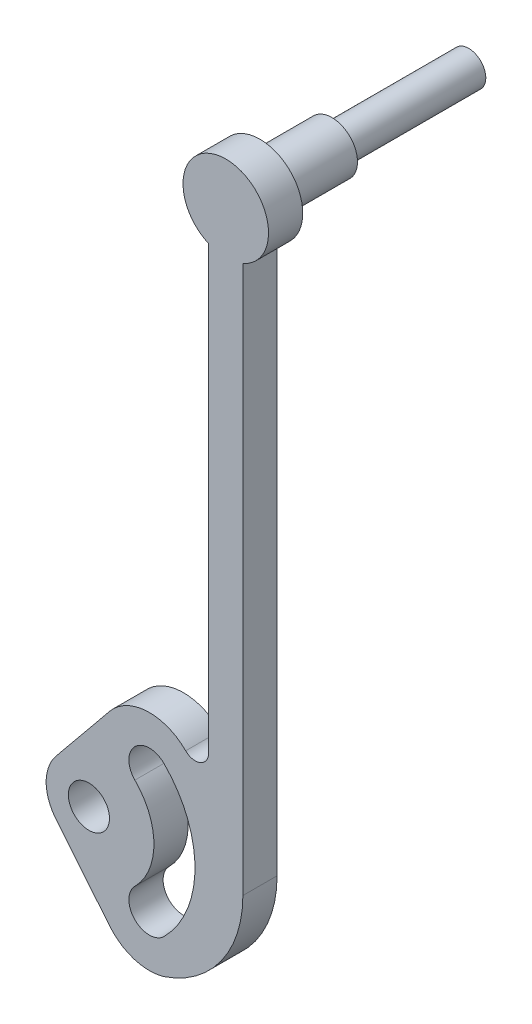
from build123d import *

# Parameters (mm, degrees)
SKETCH_1_R      = 6
EXTRUDE_1_DEPTH = 10
SKETCH_3_R      = 7.5
EXTRUDE_2_DEPTH = 21
SKETCH_4_R      = 5
EXTRUDE_3_DEPTH = 40


with BuildPart() as part:
    # 草图1 → 凸台-拉伸1 (new body)
    with BuildSketch(Plane.XY):
        with BuildLine():
            Line((-9.678413026, 7.910646073), (6.063573898, 27.170444817))
            ThreePointArc((6.063573898, 27.170444817), (16.926727904, 32.658860626), (28.284271247, 28.284271247))
            ThreePointArc((28.284271247, 28.284271247), (32.571487227, 27.431490967), (35, 31.066017178))
            Line((35, 31.066017178), (35, 160))
            ThreePointArc((35, 160), (40, 183.956439237), (45, 160))
            Line((45, 160), (45, 0))
            ThreePointArc((45, 0), (38.630100159, -19.753777039), (21.920310217, -32.0651641))
            ThreePointArc((21.920310217, -32.0651641), (13.253400527, -32.010353988), (6.063573898, -27.170444817))
            Line((6.063573898, -27.170444817), (-9.678413026, -7.910646073))
            ThreePointArc((-9.678413026, -7.910646073), (-12.5, 0), (-9.678413026, 7.910646073))
        make_face()
        Circle(SKETCH_1_R, mode=Mode.SUBTRACT)
        with BuildLine():
            ThreePointArc((21.920310217, -21.920310217), (31, 0), (21.920310217, 21.920310217))
            ThreePointArc((21.920310217, 21.920310217), (13.435028843, 21.920310217), (13.435028843, 13.435028843))
            ThreePointArc((13.435028843, 13.435028843), (19, 0), (13.435028843, -13.435028843))
            ThreePointArc((13.435028843, -13.435028843), (13.435028843, -21.920310217), (21.920310217, -21.920310217))
        make_face(mode=Mode.SUBTRACT)
    extrude(amount=EXTRUDE_1_DEPTH)

    # 草图3 → 凸台-拉伸2 (add)
    with BuildSketch(Plane(origin=(0, 0, 0), x_dir=(-1, 0, 0), z_dir=(0, 0, -1))):
        with Locations(Location((-40, 171.456439237, 0), (0, 0, 180))):
            Circle(SKETCH_3_R)
    extrude(amount=EXTRUDE_2_DEPTH)

    # 草图4 → 凸台-拉伸3 (add)
    with BuildSketch(Plane(origin=(0, 0, -21), x_dir=(-1, 0, 0), z_dir=(0, 0, -1))):
        with Locations((-40, 171.456439237)):
            Circle(SKETCH_4_R)
    extrude(amount=EXTRUDE_3_DEPTH)


solid = part.part
